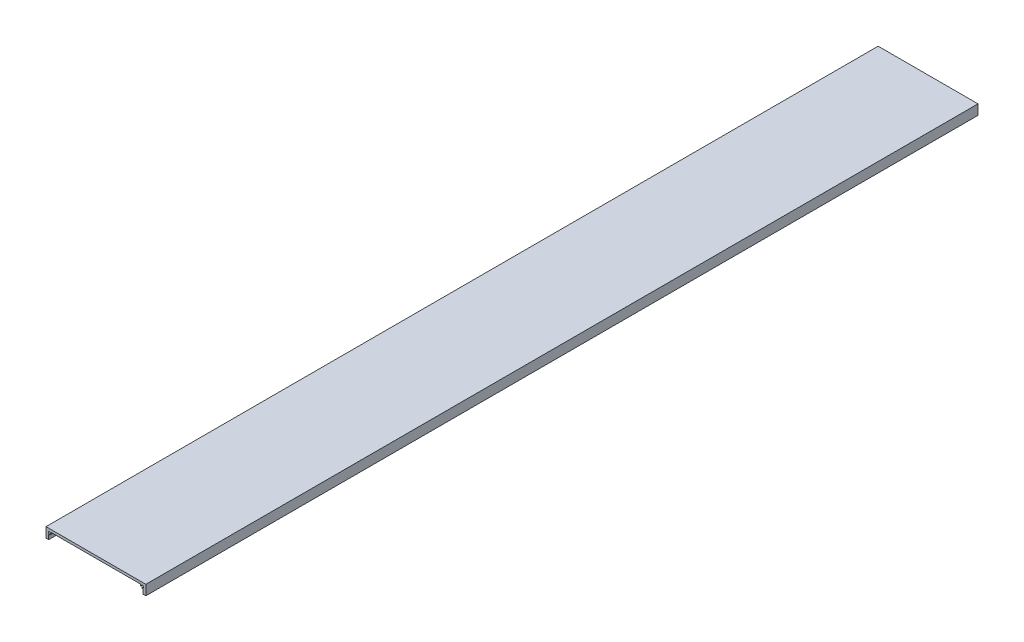
from build123d import *

# Parameters (mm, degrees)
SKETCH_1_R                  = 1.25
EXTRUDE_1_DEPTH             = 500
CUT_EXTRUDE_1_DEPTH         = 504.730086455
CUT_EXTRUDE_1_DEPTH_BACK    = 504.730086455
SKETCH_2_W                  = 1.7
SKETCH_2_H                  = 1.9
HOLE_WIZARD_M3_1_AT_2_COUNT = 2
HOLE_WIZARD_M3_1_AT_2_PITCH = 112


with BuildPart() as part:
    # 草图1 → 凸台-拉伸1 (new, symmetric)
    with BuildSketch(Plane.XY):
        Polygon((60, 12), (-60, 12), (-60, 0), (-56.8, 0), (-56.8, 5.5), (-53.7, 5.5), (-53.7, 9), (53.7, 9), (53.7, 5.5), (56.8, 5.5), (56.8, 0), (60, 0), align=None)
        with Locations((-56, 7.7)):
            Circle(SKETCH_1_R, mode=Mode.SUBTRACT)
        with Locations(Location((56, 7.7, 0), (0, 0, 180))):
            Circle(SKETCH_1_R, mode=Mode.SUBTRACT)
    extrude(amount=EXTRUDE_1_DEPTH, both=True)

    # 草图2 → 切除-拉伸1 (cut, two sides: drawn at the far end of the back side and taken through both)
    with BuildSketch(Plane.XY.offset(-CUT_EXTRUDE_1_DEPTH_BACK)):
        with Locations((-54.55, 6.45)):
            Rectangle(SKETCH_2_W, SKETCH_2_H)
        with Locations((54.55, 6.45)):
            Rectangle(SKETCH_2_W, SKETCH_2_H)
    extrude(amount=CUT_EXTRUDE_1_DEPTH + CUT_EXTRUDE_1_DEPTH_BACK, mode=Mode.SUBTRACT)

    # 草图7 → M3 螺纹孔1 (revolve, cut)
    with BuildSketch(Plane(origin=(-56, 7.7, 500), x_dir=(0, -1, 0), z_dir=(1, 0, 0))):
        Polygon((0, 0), (0, 20.781118805), (1.3, 20), (1.3, 0), align=None)
    hole_wizard_m3_1 = revolve(axis=Axis((-56, 7.7, 506.35), (0, 0, -1)), mode=Mode.SUBTRACT)

    # M3 螺纹孔1 at 2: M3 螺纹孔1 ×2
    with Locations(*[(i * HOLE_WIZARD_M3_1_AT_2_PITCH, 0, 0) for i in range(1, HOLE_WIZARD_M3_1_AT_2_COUNT)]):
        add(hole_wizard_m3_1, mode=Mode.SUBTRACT)

    # 镜向1: M3 螺纹孔1 across plane
    add(hole_wizard_m3_1.mirror(Plane.XY), mode=Mode.SUBTRACT)

    # 镜向1 copy 1 sketch → 镜向1 copy 1 (revolve, cut)
    with BuildSketch(Plane(origin=(56, 7.7, -500), x_dir=(0, -1, 0), z_dir=(1, 0, 0))):
        Polygon((0, 0), (0, -20.781118805), (1.3, -20), (1.3, 0), align=None)
    revolve(axis=Axis((56, 7.7, -506.35), (0, 0, -1)), mode=Mode.SUBTRACT)


solid = part.part
